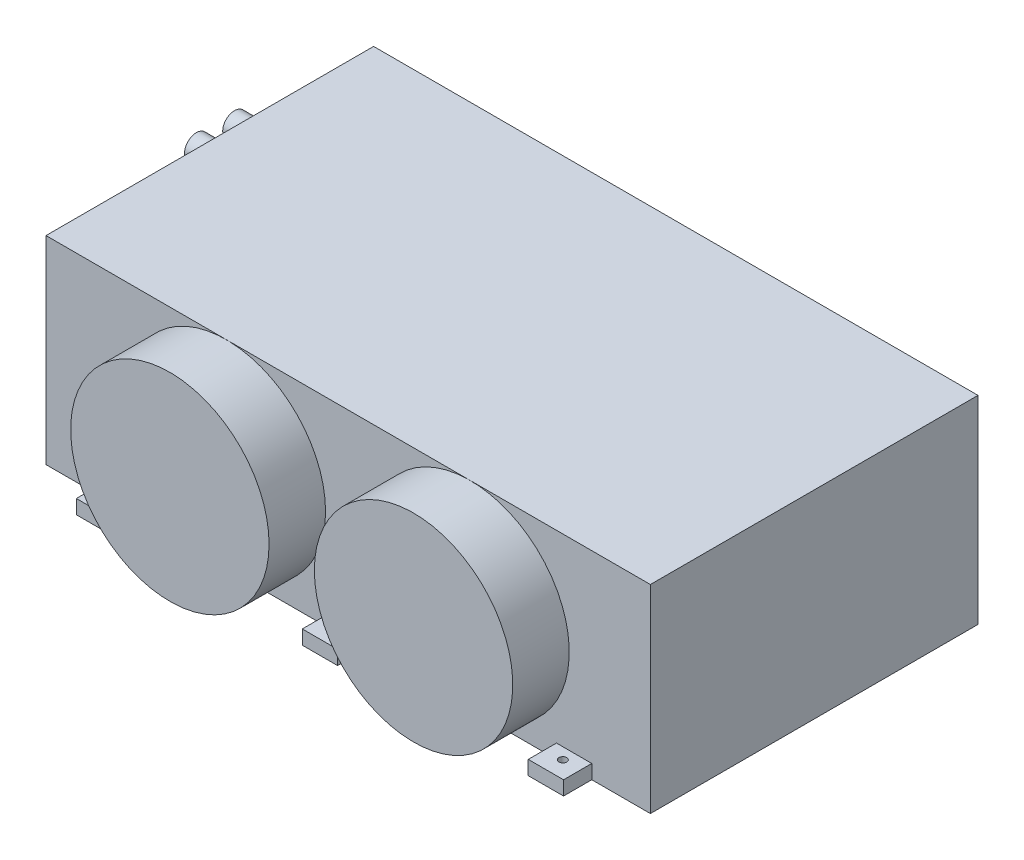
SolidWorks part; units mm, degrees
material "SPCC冷轧板喷塑"
ref_plane "前视基准面" through (0, 0, 0) normal (0, 0, 1) x (1, 0, 0)
ref_plane "上视基准面" through (0, 0, 0) normal (0, 1, 0) x (1, 0, 0)
ref_plane "右视基准面" through (0, 0, 0) normal (1, 0, 0) x (0, 0, -1)
other "Configuration Table"
sketch "草图1" plane through (0, 0, 0) normal (0, 1, 0) x (1, 0, 0)
  line L1 (428, -232) -> (-428, -232)
  line L2 (428, -232) -> (428, 232)
  line L3 (428, 232) -> (-428, 232)
  line L4 (-428, -232) -> (-428, 232)
  line L5 (428, -232) -> (-428, 232) construction
  line L6 (428, 232) -> (-428, -232) construction
  point P0 (0, 0)
  dimension "D1" = 856
  dimension "D2" = 464
extrude "凸台-拉伸1" add sketch "草图1" along normal blind 281
sketch "草图3" plane through (0, 0, 0) normal (0, -1, 0) x (1, 0, 0)
  line L0 (-428, 232) -> (428, 232) construction
  line L1 (-25, 272) -> (25, 272)
  line L2 (-25, 272) -> (-25, 232)
  line L3 (-25, 232) -> (25, 232)
  line L4 (25, 272) -> (25, 232)
  dimension "D1" = 40
  dimension "D2" = 50
  dimension "D3" = 25
extrude "凸台-拉伸2" add sketch "草图3" against normal blind 20 separate body
mirror "镜向1" about plane through (0, 0, 0) normal (0, 0, 1) of bodies 108
pattern_linear "阵列(线性)2" count 2 spacing 320 along (1, 0, 0) of bodies 108 109
mirror "镜向2" about plane through (0, 0, 0) normal (1, 0, 0) of bodies 111 112
sketch "草图4" plane through (0, 20, 0) normal (0, 1, 0) x (1, 0, 0)
  line L0 (-320, 248) -> (0, 248) construction
  line L1 (-320, 248) -> (-320, -248) construction
  circle A0 centre (-320, 248) radius 5.5
  circle A1 centre (0, 248) radius 5.5
  circle A2 centre (320, 248) radius 5.5
  circle A3 centre (0, -248) radius 5.5
  circle A4 centre (320, -248) radius 5.5
  circle A5 centre (-320, -248) radius 5.5
  dimension "D1" = 11
  dimension "D2" = 320
  dimension "D3" = 248
  dimension "D6" = 320
  dimension "D7" = 496
  dimension "D4" = 3
  dimension "D5" = 2
extrude "切除-拉伸1" cut sketch "草图4" against normal through all
sketch "草图5" plane through (0, 0, 232) normal (0, 0, 1) x (1, 0, 0)
  circle A0 centre (-172.5575, 140.5) radius 140.5
extrude "凸台-拉伸3" add sketch "草图5" along normal blind 80 separate body
mirror "镜向3" about plane through (0, 0, 0) normal (1, 0, 0) of bodies 121
sketch "草图6" plane through (-428, 0, 0) normal (-1, 0, 0) x (0, 0, 1)
  line L0 (-232, 281) -> (-232, 0) construction
  line L2 (-232, 0) -> (-272, 0) construction
  circle A0 centre (-69.5, 249.5) radius 16.75
  circle A1 centre (-69.5, 249.5) radius 13.25
  dimension "D1" = 33.5
  dimension "D2" = 162.5
  dimension "D3" = 249.5
  dimension "D4" = 3.5
extrude "凸台-拉伸4" add sketch "草图6" along normal blind 34.5 separate body
pattern_linear "阵列(线性)3" count 2 spacing 54 along (0, 0, 1) of bodies 123
